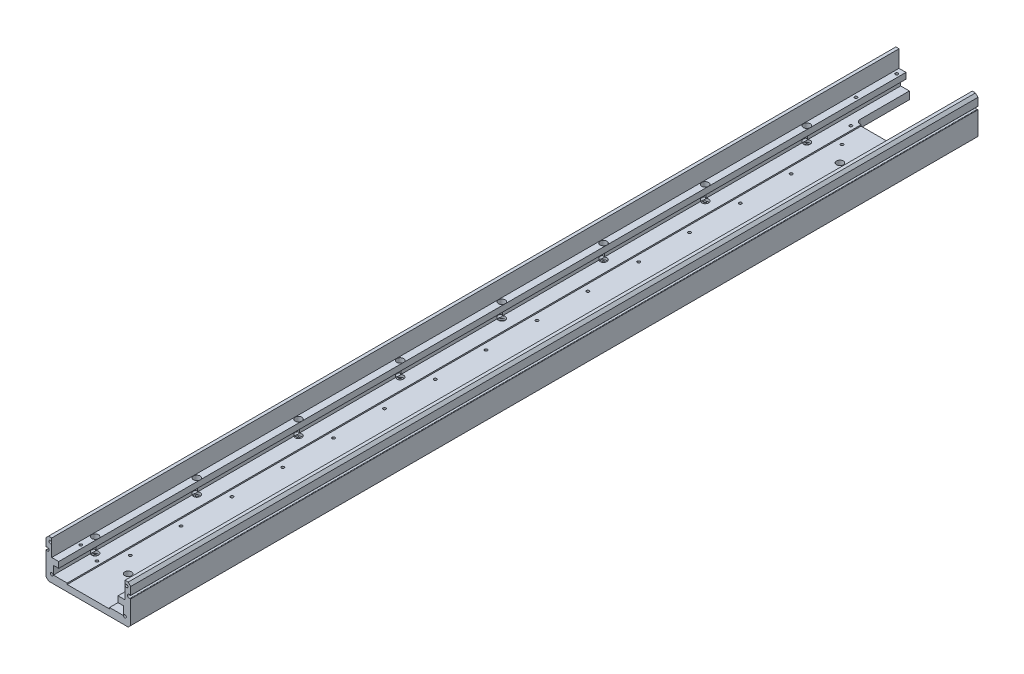
SolidWorks part; units mm, degrees
material "6061 合金"
ref_plane "前视基准面" through (0, 0, 0) normal (0, 0, 1) x (1, 0, 0)
ref_plane "上视基准面" through (0, 0, 0) normal (0, 1, 0) x (1, 0, 0)
ref_plane "右视基准面" through (0, 0, 0) normal (1, 0, 0) x (0, 0, -1)
sketch "草图1" plane through (0, 0, 0) normal (0, 0, 1) x (1, 0, 0)
  line L1 (-50, 23) -> (50, 23)
  line L2 (-50, 23) -> (-50, -23)
  line L3 (-50, -23) -> (50, -23)
  line L4 (50, 23) -> (50, -23)
  line L5 (-50, 23) -> (50, -23) construction
  line L6 (-50, -23) -> (50, 23) construction
  point P0 (0, 0)
  dimension "D1" = 100
  dimension "D2" = 46
extrude "凸台-拉伸1" add sketch "草图1" along normal mid plane 1000
chamfer "倒角1" distance 3 angle 45 4 edges at (50, 23, 0) (50, -23, 0) (-50, 23, 0) (-50, -23, 0)
sketch "草图2" plane through (0, 0, 0) normal (0, 0, 1) x (1, 0, 0)
  line L0 (0, 23) -> (0, -23) construction
  line L1 (47, 23) -> (-47, 23) construction
  line L2 (-47, -23) -> (47, -23) construction
  line L3 (43.25, 23) -> (-43.25, 23)
  line L4 (-43.25, 23) -> (-43.25, 3)
  line L5 (-43.25, 3) -> (-35, 3)
  line L6 (-35, 3) -> (-35, -4)
  line L7 (-35, -4) -> (-41.25, -4)
  line L8 (-41.25, -4) -> (-41.25, -14)
  line L9 (-41.25, -14) -> (-25, -14)
  line L10 (-25, -14) -> (-25, -15.5)
  line L11 (-25, -15.5) -> (25, -15.5)
  line L12 (43.25, 23) -> (43.25, 3)
  line L13 (43.25, 3) -> (35, 3)
  line L14 (35, 3) -> (35, -4)
  line L15 (35, -4) -> (41.25, -4)
  line L16 (41.25, -4) -> (41.25, -14)
  line L17 (41.25, -14) -> (25, -14)
  line L18 (25, -14) -> (25, -15.5)
  point P23 (0, -15.5)
  dimension "D1" = 50
  dimension "D2" = 7.5
  dimension "D3" = 9
  dimension "D4" = 82.5
  dimension "D5" = 70
  dimension "D6" = 86.5
  dimension "D7" = 10
  dimension "D8" = 7
extrude "切除-拉伸1" cut sketch "草图2" against normal through all both and the other way through all
sketch "草图3" plane through (0, 0, 0) normal (0, 0, 1) x (1, 0, 0)
  line L0 (0, -25.5404) -> (0, 0) construction
  line L1 (-47, -23) -> (47, -23) construction
  circle A0 centre (-43.15, -14) radius 1.6
  circle A1 centre (-45, 18) radius 1.6
  circle A2 centre (43.15, -14) radius 1.6
  circle A3 centre (45, 18) radius 1.6
  dimension "D2" = 86.3
  dimension "D3" = 3.2
  dimension "D4" = 32
  dimension "D1" = 9
  dimension "D5" = 90
extrude "切除-拉伸2" cut sketch "草图3" against normal through all both and the other way through all
sketch "草图4" plane through (0, 0, 0) normal (0, 0, 1) x (1, 0, 0)
  line L0 (0, 0) -> (0, -23.0913) construction
  line L1 (-43.25, 23) -> (-47, 23) construction
  line L2 (-50, 20) -> (-50, -20) construction
  circle A0 centre (-48.2, 9.1) radius 2
  circle A1 centre (48.2, 9.1) radius 2
  dimension "D2" = 1.8
  dimension "D3" = 4
  dimension "D1" = 13.9
extrude "切除-拉伸3" cut sketch "草图4" against normal through all both and the other way through all
sketch "草图5" plane through (0, -23, 0) normal (0, -1, 0) x (1, 0, 0)
  line L0 (0, -500) -> (0, 500) construction
  line L1 (-47, -500) -> (47, -500) construction
  line L2 (-47, 500) -> (47, 500) construction
  line L4 (-31, -437) -> (31, -437)
  line L5 (-31, -437) -> (-31, -500)
  line L6 (-31, -500) -> (31, -500)
  line L7 (31, -437) -> (31, -500)
  line L8 (-31, -437) -> (31, -500) construction
  line L9 (-31, -500) -> (31, -437) construction
  point P6 (0, -468.5)
  dimension "D1" = 62
  dimension "D2" = 63
extrude "切除-拉伸4" cut sketch "草图5" against normal through all
hole_wizard "M5 螺纹孔1" positions "草图7" profile "草图6" tap size "M5" standard "GB"
sketch "草图7" plane through (0, 0, 400) normal (0, 0, 1) x (1, 0, 0)
  line L0 (-43.15, -14) -> (-43.15, 0) construction
  line L5 (-35, -0.5) -> (-43.15, -0.5) construction
  line L6 (-35, 3) -> (-35, -4) construction
  point P20 (-43.15, -0.5)
sketch "草图6" plane through (-43.15, -0.5, 400) normal (1, 0, 0) x (0, -1, 0)
  line L0 (0, 0) -> (0, 16.2618)
  line L1 (0, 16.2618) -> (2.1, 15)
  line L2 (2.1, 15) -> (2.1, 0)
  line L5 (2.1, 0) -> (0, 0)
  line L10 (0, 16.2618) -> (-2.1, 15) construction
  line L11 (0, -6.35) -> (0, 107.95) construction
  dimension "螺纹孔钻头直径" = 4.2
  dimension "螺纹孔钻头深度" = 15
  dimension "导头角度" = 118
cosmetic thread "孔螺蚊线1" [suppressed] parameters "D1"=15, "D2"=5
mirror "镜向1" [suppressed] about plane through (0, 0, 0) normal (1, 0, 0)
mirror "镜向2" [suppressed] about plane through (0, 0, 0) normal (0, 0, 1)
hole_wizard "M4 螺纹孔1" positions "草图9" profile "草图8" tap size "M4" standard "GB"
sketch "草图9" plane through (0, 0, 500) normal (0, 0, 1) x (1, 0, 0)
  point P0 (-43.15, -14)
  point P3 (-45, 18)
  point P6 (45, 18)
  point P9 (43.15, -14)
sketch "草图8" plane through (-43.15, -14, 500) normal (1, 0, 0) x (0, -1, 0)
  line L0 (0, 0) -> (0, 12.9914)
  line L1 (0, 12.9914) -> (1.65, 12)
  line L2 (1.65, 12) -> (1.65, 0)
  line L5 (1.65, 0) -> (0, 0)
  line L10 (0, 12.9914) -> (-1.65, 12) construction
  line L11 (0, -6.35) -> (0, 107.95) construction
  dimension "螺纹孔钻头直径" = 3.3
  dimension "螺纹孔钻头深度" = 12
  dimension "导头角度" = 118
cosmetic thread "孔螺蚊线2" parameters "D1"=10, "D2"=4
cosmetic thread "孔螺蚊线3" parameters "D1"=10, "D2"=4
cosmetic thread "孔螺蚊线4" parameters "D1"=10, "D2"=4
cosmetic thread "孔螺蚊线5" parameters "D1"=10, "D2"=4
mirror "镜向3" about plane through (0, 0, 0) normal (0, 0, 1) of "M4 螺纹孔1"
fillet "圆角1" radius 5 2 edges at (31, -18.5, -437) (-31, -18.5, -437)
hole_wizard "M4 螺纹孔2" positions "草图11" profile "草图10" tap size "M4" standard "GB"
sketch "草图11" plane through (0, 3, 0) normal (0, 1, 0) x (1, 0, 0)
  line L0 (-39, 493) -> (-39, 445) construction
  line L1 (-39, 445) -> (-39, -470) construction
  line L3 (-43.25, -500) -> (-35, -500) construction
  line L4 (-43.25, 500) -> (-35, 500) construction
  point P0 (-39, 493)
  point P2 (-39, 445)
  point P4 (-39, -470)
  dimension "D1" = 30
  dimension "D2" = 7
  dimension "D3" = 48
  dimension "D4" = 39
sketch "草图10" plane through (-39, 3, -493) normal (1, 0, 0) x (0, 0, 1)
  line L0 (0, 0) -> (0, 26)
  line L1 (0, 26) -> (1.65, 26)
  line L2 (1.65, 26) -> (1.65, 0)
  line L5 (1.65, 0) -> (0, 0)
  line L11 (0, -6.35) -> (0, 20.821) construction
  dimension "通孔螺纹孔钻头直径" = 3.3
  dimension "通孔螺纹孔钻头深度" = 26
cosmetic thread "孔螺蚊线6" parameters "D2"=4
cosmetic thread "孔螺蚊线7" parameters "D2"=4
cosmetic thread "孔螺蚊线8" parameters "D2"=4
mirror "镜向4" about plane through (0, 0, 0) normal (1, 0, 0) of "M4 螺纹孔2"
fillet "圆角2" radius 0.35 4 edges at (-50, 8.2282, 0) (-50, 9.9718, 0) (50, 9.9718, 0) (50, 8.2282, 0)
hole_wizard "M4 螺纹孔3" positions "草图13" profile "草图12" tap size "M4" standard "GB" end condition through all
sketch "草图13" plane through (0, -15.5, 0) normal (0, 1, 0) x (1, 0, 0)
  line L0 (-17.5, 407) -> (17.5, 407) construction
  line L3 (0, 407) -> (0, 437) construction
  line L4 (25, 437) -> (-25, 437) construction
  point P0 (17.5, 407)
  point P3 (-17.5, 407)
  dimension "D1" = 35
  dimension "D2" = 30
sketch "草图12" plane through (17.5, -15.5, -407) normal (1, 0, 0) x (0, 0, 1)
  line L0 (0, 0) -> (0, 7.5)
  line L1 (0, 7.5) -> (1.65, 7.5)
  line L2 (1.65, 7.5) -> (1.65, 0)
  line L5 (1.65, 0) -> (0, 0)
  line L11 (0, -6.35) -> (0, 107.95) construction
  dimension "通孔螺纹孔钻头直径" = 3.3
  dimension "通孔螺纹孔钻头深度" = 7.5
cosmetic thread "孔螺蚊线34" parameters "D2"=4
cosmetic thread "孔螺蚊线35" parameters "D2"=4
pattern_linear "阵列(线性)1" count 15 spacing 60 along (0, 0, 1) of "M4 螺纹孔3"
sketch "草图14" plane through (0, -23, 0) normal (0, -1, 0) x (1, 0, 0)
  line L0 (-47, 500) -> (47, 500) construction
  line L1 (-35, 601.9002) -> (35, 601.9002)
  line L2 (-35, 601.9002) -> (-35, 425)
  line L3 (-35, 425) -> (35, 425)
  line L4 (35, 601.9002) -> (35, 425)
  line L5 (-35, 601.9002) -> (35, 425) construction
  line L6 (-35, 425) -> (35, 601.9002) construction
  point P0 (0, 513.4501)
  dimension "D1" = 70
  dimension "D2" = 75
extrude "切除-拉伸5" [suppressed] cut sketch "草图14" against normal through all
fillet "圆角3" [suppressed] radius 5
hole_wizard "打孔尺寸(%根据)开槽圆柱头螺钉的类型2" positions "草图16" profile "草图17" counterbore size "M4" standard "GB" end condition through all
sketch "草图16" plane through (0, 3, 0) normal (0, 1, 0) x (1, 0, 0)
  line L0 (0, 0) -> (0, 406.8475) construction
  line L2 (25, 437) -> (-25, 437) construction
  point P0 (-39, 387)
  point P2 (39, 387)
  dimension "D1" = 78
  dimension "D2" = 50
sketch "草图17" plane through (-39, 3, -387) normal (1, 0, 0) x (0, 0, 1)
  line L0 (0, 0) -> (0, 26)
  line L1 (0, 26) -> (2.25, 26)
  line L3 (2.25, 26) -> (2.25, 20)
  line L4 (2.25, 20) -> (3.995, 20)
  line L5 (3.995, 20) -> (3.995, 0)
  line L7 (3.995, 0) -> (0, 0)
  line L11 (0, -6.35) -> (0, 107.95) construction
  dimension "通孔孔直径" = 4.5
  dimension "通孔孔深度" = 26
  dimension "柱形沉头孔直径" = 7.99
  dimension "柱形沉头孔深度" = 20
pattern_linear "阵列(线性)2" count 8 spacing 120 along (0, 0, 1) of "打孔尺寸(%根据)开槽圆柱头螺钉的类型2"
hole_wizard "M4 螺纹孔4" positions "草图23" profile "草图24" tap size "M4" standard "GB" end condition through all
sketch "草图23" plane through (0, -14, 0) normal (0, 1, 0) x (1, 0, 0)
  line L0 (0, 437) -> (0, 374.849) construction
  line L1 (25, 437) -> (-25, 437) construction
  point P0 (30, 430)
  point P2 (-30, 430)
  dimension "D1" = 60
  dimension "D2" = 7
sketch "草图24" plane through (30, -14, -430) normal (1, 0, 0) x (0, 0, 1)
  line L0 (0, 0) -> (0, 9)
  line L1 (0, 9) -> (1.65, 9)
  line L2 (1.65, 9) -> (1.65, 0)
  line L5 (1.65, 0) -> (0, 0)
  line L11 (0, -6.35) -> (0, 107.95) construction
  dimension "通孔螺纹孔钻头直径" = 3.3
  dimension "通孔螺纹孔钻头深度" = 9
cosmetic thread "孔螺蚊线36" parameters "D2"=4
cosmetic thread "孔螺蚊线37" parameters "D2"=4
pattern_linear "阵列(线性)4" count 2 spacing 890 along (0, 0, 1) of "M4 螺纹孔4"
sketch "草图25" plane through (0, -15.5, 0) normal (0, 1, 0) x (1, 0, 0)
  line L0 (-39, -453) -> (39, -453) construction
  line L1 (-39, 387) -> (39, 387) construction
  circle A0 centre (0, -453) radius 4
  circle A1 centre (0, 387) radius 4
  point P8 (0, 387)
  point P9 (0, -453)
  dimension "D1" = 8
extrude "切除-拉伸6" cut sketch "草图25" against normal blind 10
